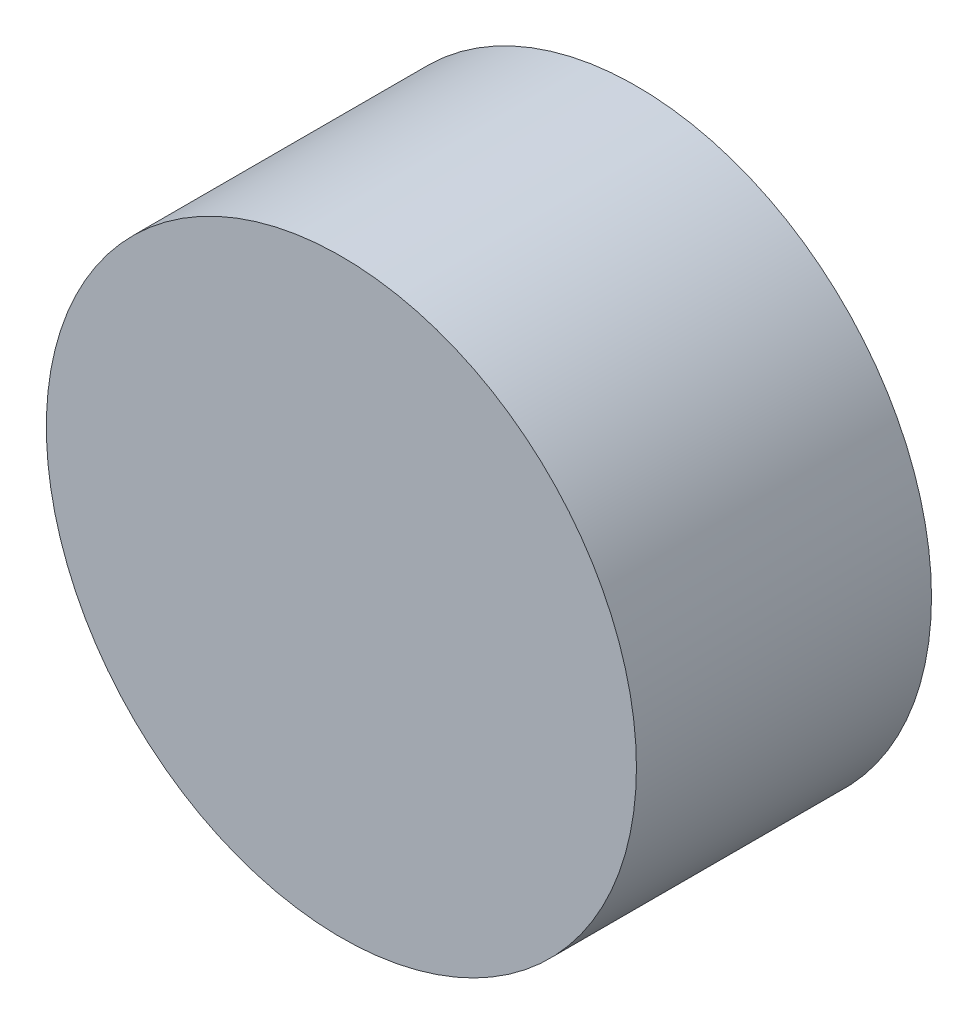
SolidWorks part; units mm, degrees
ref_plane "Front Plane" through (0, 0, 0) normal (0, 0, 1) x (1, 0, 0)
ref_plane "Top Plane" through (0, 0, 0) normal (0, 1, 0) x (1, 0, 0)
ref_plane "Right Plane" through (0, 0, 0) normal (1, 0, 0) x (0, 0, -1)
sketch "Sketch1" plane through (0, 0, 0) normal (0, 0, 1) x (1, 0, 0)
  circle A0 centre (0, 0) radius 6.35
  dimension "D1" = 12.7
extrude "Boss-Extrude1" add sketch "Sketch1" along normal blind 6.35
sketch "Sketch2" plane through (0, 0, 6.35) normal (0, 0, 1) x (1, 0, 0)
  circle A0 centre (0, 0) radius 1
  dimension "D1" = 2
sketch "Sketch3" plane through (0, 0, 0) normal (0, 1, 0) x (1, 0, 0)
  line L0 (0, -6.35) -> (0, -8.35)
  dimension "D1" = 2
sketch "Sketch5" plane through (0, 0, 0) normal (0, 0, -1) x (-1, 0, 0)
  circle A0 centre (0, 0) radius 1.1759
